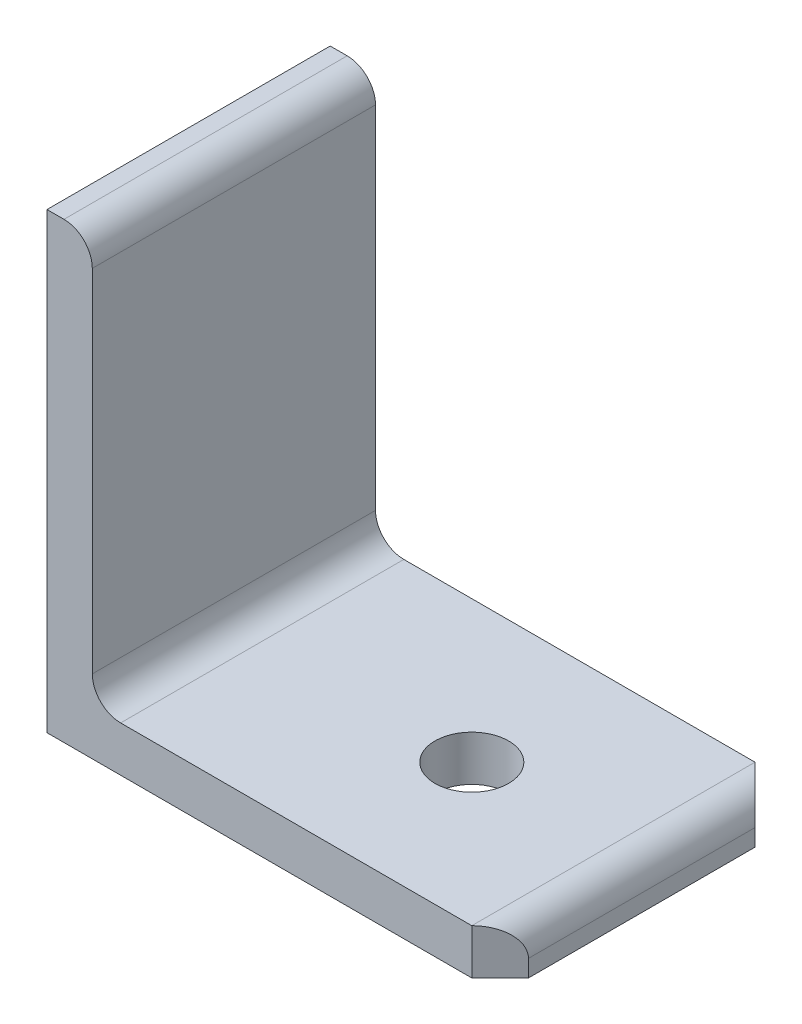
SolidWorks part; units mm, degrees
material "1023 碳钢板 (SS)"
ref_plane "前视基准面" through (0, 0, 0) normal (0, 0, 1) x (1, 0, 0)
ref_plane "上视基准面" through (0, 0, 0) normal (0, 1, 0) x (1, 0, 0)
ref_plane "右视基准面" through (0, 0, 0) normal (1, 0, 0) x (0, 0, -1)
sketch "草图1" plane through (0, 0, 0) normal (0, 0, 1) x (1, 0, 0)
  line L0 (0, 0) -> (0, -80)
  line L1 (0, -80) -> (80, -80)
  line L2 (8, 0) -> (8, -72)
  line L3 (8, -72) -> (80, -72)
  line L4 (8, 0) -> (0, 0)
  line L5 (80, -72) -> (80, -80)
  dimension "D1" = 80
  dimension "D2" = 80
  dimension "D3" = 8
extrude "凸台-拉伸1" add sketch "草图1" along normal blind 50 contours L5 L1 L0 L4 L2 L3
sketch "草图2" plane through (0, -72, 0) normal (0, 1, 0) x (1, 0, 0)
  line L0 (8, 0) -> (80, 0) construction
  line L1 (80, -50) -> (80, 0) construction
  circle A0 centre (50, -25) radius 6.5
  dimension "D1" = 25
  dimension "D2" = 30
  dimension "D3" = 13
extrude "切除-拉伸1" cut sketch "草图2" against normal blind 50
fillet "圆角1" radius 5 1 edges at (8, -72, 25)
fillet "圆角2" radius 5 1 edges at (8, 0, 25)
chamfer "倒角1" distance 5 angle 45 2 edges at (80, -76, 0) (80, -76, 50)
fillet "圆角3" radius 5 1 edges at (80, -72, 25)
